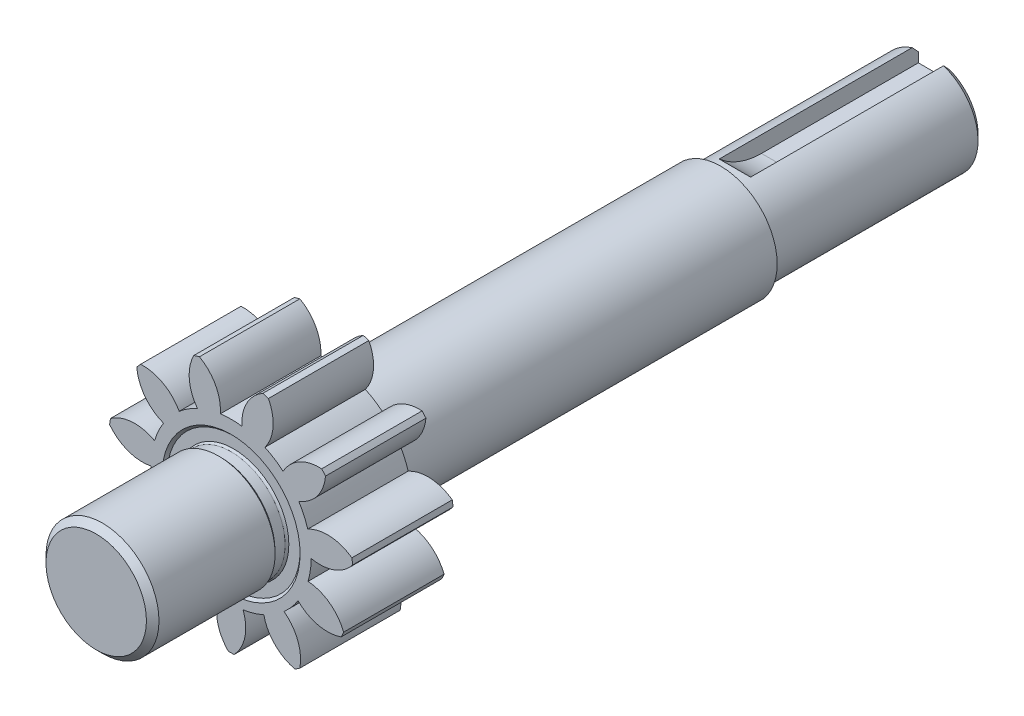
from build123d import *

# Parameters (mm, degrees)
EXTRUDE_1_DEPTH     = 16
SKETCH_2_R          = 9
EXTRUDE_2_DEPTH     = 21.5
EXTRUDE_START       = 62
SKETCH_3_R          = 9
EXTRUDE_3_DEPTH     = 62
SKETCH_4_R          = 8
EXTRUDE_4_DEPTH     = 34
CUT_EXTRUDE_1_DEPTH = 2.5
CHAMFER_1_SIZE      = 1


with BuildPart() as part:
    # 草图1 → 凸台-拉伸1 (new body)
    with BuildSketch(Plane.XY):
        with BuildLine():
            ThreePointArc((-17.539719795, -8.188913461), (-13.882626521, -8.407262966), (-10.672515451, -6.641705083))
            ThreePointArc((-10.672515451, -6.641705083), (-9.635051323, -8.016686689), (-8.421711588, -9.239271212))
            ThreePointArc((-8.421711588, -9.239271212), (-10.626145075, -12.165442895), (-10.930476691, -15.816386607))
            ThreePointArc((-10.930476691, -15.816386607), (-10.54249594, -16.072311082), (-10.148525822, -16.318915917))
            ThreePointArc((-10.148525822, -16.318915917), (-6.95393453, -14.525429313), (-5.207949909, -11.304630433))
            ThreePointArc((-5.207949909, -11.304630433), (-3.591808367, -11.900443112), (-1.910102932, -12.272965675))
            ThreePointArc((-1.910102932, -12.272965675), (-2.18258254, -15.926424664), (-0.464753394, -19.162328053))
            ThreePointArc((-0.464753394, -19.162328053), (0, -19.167867192), (0.464753394, -19.162328053))
            ThreePointArc((0.464753394, -19.162328053), (2.18258254, -15.926424664), (1.910102932, -12.272965675))
            ThreePointArc((1.910102932, -12.272965675), (3.591808367, -11.900443112), (5.207949909, -11.304630433))
            ThreePointArc((5.207949909, -11.304630433), (6.95393453, -14.525429313), (10.148525822, -16.318915917))
            ThreePointArc((10.148525822, -16.318915917), (10.54249594, -16.072311082), (10.930476691, -15.816386607))
            ThreePointArc((10.930476691, -15.816386607), (10.626145075, -12.165442895), (8.421711588, -9.239271212))
            ThreePointArc((8.421711588, -9.239271212), (9.635051323, -8.016686689), (10.672515451, -6.641705083))
            ThreePointArc((10.672515451, -6.641705083), (13.882626521, -8.407262966), (17.539719795, -8.188913461))
            ThreePointArc((17.539719795, -8.188913461), (17.737823909, -7.768459945), (17.925850869, -7.343404347))
            ThreePointArc((17.925850869, -7.343404347), (15.69598163, -4.436569144), (12.25948632, -3.166723601))
            ThreePointArc((12.25948632, -3.166723601), (12.619233563, -1.482239065), (12.748632746, 0.235364522))
            ThreePointArc((12.748632746, 0.235364522), (16.403682682, 0.485599789), (19.362176663, 2.646460979))
            ThreePointArc((19.362176663, 2.646460979), (19.301518117, 3.107272155), (19.229894055, 3.566506728))
            ThreePointArc((19.229894055, 3.566506728), (15.782454919, 4.806333783), (12.204960767, 4.016686199))
            ThreePointArc((12.204960767, 4.016686199), (11.596898309, 5.628258809), (10.777149222, 7.143157375))
            ThreePointArc((10.777149222, 7.143157375), (13.716685494, 9.329737862), (15.037279247, 12.747052577))
            ThreePointArc((15.037279247, 12.747052577), (14.7371167, 13.10191712), (14.42858175, 13.449526936))
            ThreePointArc((14.42858175, 13.449526936), (10.858110285, 12.628709513), (8.275446406, 10.030276331))
            ThreePointArc((8.275446406, 10.030276331), (6.892629782, 11.057274099), (5.383996967, 11.888498053))
            ThreePointArc((5.383996967, 11.888498053), (6.674737579, 15.317199905), (5.938151919, 18.905994868))
            ThreePointArc((5.938151919, 18.905994868), (5.493784858, 19.042245794), (5.046296687, 19.167867192))
            ThreePointArc((5.046296687, 19.167867192), (2.486392356, 16.547009024), (1.718536283, 12.964774418))
            ThreePointArc((1.718536283, 12.964774418), (0, 13.081132808), (-1.718536283, 12.964774418))
            ThreePointArc((-1.718536283, 12.964774418), (-2.486392356, 16.547009024), (-5.046296687, 19.167867192))
            ThreePointArc((-5.046296687, 19.167867192), (-5.493784858, 19.042245794), (-5.938151919, 18.905994868))
            ThreePointArc((-5.938151919, 18.905994868), (-6.674737579, 15.317199905), (-5.383996967, 11.888498053))
            ThreePointArc((-5.383996967, 11.888498053), (-6.892629782, 11.057274099), (-8.275446406, 10.030276331))
            ThreePointArc((-8.275446406, 10.030276331), (-10.858110285, 12.628709513), (-14.42858175, 13.449526936))
            ThreePointArc((-14.42858175, 13.449526936), (-14.7371167, 13.10191712), (-15.037279247, 12.747052577))
            ThreePointArc((-15.037279247, 12.747052577), (-13.716685494, 9.329737862), (-10.777149222, 7.143157375))
            ThreePointArc((-10.777149222, 7.143157375), (-11.596898309, 5.628258809), (-12.204960767, 4.016686199))
            ThreePointArc((-12.204960767, 4.016686199), (-15.782454919, 4.806333783), (-19.229894055, 3.566506728))
            ThreePointArc((-19.229894055, 3.566506728), (-19.301518117, 3.107272155), (-19.362176663, 2.646460979))
            ThreePointArc((-19.362176663, 2.646460979), (-16.403682682, 0.485599789), (-12.748632746, 0.235364522))
            ThreePointArc((-12.748632746, 0.235364522), (-12.619233563, -1.482239065), (-12.25948632, -3.166723601))
            ThreePointArc((-12.25948632, -3.166723601), (-15.69598163, -4.436569144), (-17.925850869, -7.343404347))
            ThreePointArc((-17.925850869, -7.343404347), (-17.737823909, -7.768459945), (-17.539719795, -8.188913461))
        make_face()
    extrude(amount=EXTRUDE_1_DEPTH)

    # 草图2 → 凸台-拉伸2 (add)
    with BuildSketch(Plane.XY.offset(16)):
        Circle(SKETCH_2_R)
    extrude(amount=EXTRUDE_2_DEPTH)

    # 草图3 → 凸台-拉伸3 (add)
    with BuildSketch(Plane(origin=(0, 0, 0), x_dir=(-1, 0, 0), z_dir=(0, 0, -1)).offset(EXTRUDE_START)):
        with Locations(Location((0, 0, 0), (0, 0, 180))):
            Circle(SKETCH_3_R)
    extrude(amount=-EXTRUDE_3_DEPTH)

    # 草图4 → 凸台-拉伸4 (add)
    with BuildSketch(Plane(origin=(0, 0, -62), x_dir=(-1, 0, 0), z_dir=(0, 0, -1))):
        Circle(SKETCH_4_R)
    extrude(amount=EXTRUDE_4_DEPTH)

    # 草图5 → 切除-旋转1 (revolve, cut)
    with BuildSketch(Plane(origin=(0, 0, 0), x_dir=(0, 0, -1), z_dir=(1, 0, 0)), mode=Mode.PRIVATE) as cut_revolve_1_sk:
        with BuildLine():
            Line((-16, 10.9894116), (-15.6, 10.5894116))
            Line((-15.6, 10.5894116), (-15.6, 8.792688481))
            ThreePointArc((-15.6, 8.792688481), (-15.785456972, 8.662432859), (-16, 8.5894116))
            Line((-16, 8.5894116), (-17.6, 8.5894116))
            Line((-17.6, 8.5894116), (-18, 8.9894116))
            Line((-18, 8.9894116), (-18, 10.9894116))
            Line((-18, 10.9894116), (-16, 10.9894116))
        make_face()
    cut_revolve_1 = revolve(cut_revolve_1_sk.sketch.rotate(Axis((0, 0, 37.5), (0, 0, -1)), 90), axis=Axis((0, 0, 37.5), (0, 0, -1)), mode=Mode.SUBTRACT)

    # 镜向1: 切除-旋转1 across plane
    add(cut_revolve_1.mirror(Plane.XY.offset(8)), mode=Mode.SUBTRACT)

    # 草图6 → 切除-拉伸1 (cut, symmetric)
    with BuildSketch(Plane(origin=(0, 0, 0), x_dir=(0, 0, -1), z_dir=(1, 0, 0))):
        with BuildLine():
            Line((96, 12.940111189), (96, 5))
            Line((96, 5), (71, 5))
            ThreePointArc((71, 5), (64.570358548, 7.341037224), (61.151123092, 13.268057839))
            Line((61.151123092, 13.268057839), (61.151123092, 20.241558611))
            Line((61.151123092, 20.241558611), (96, 20.241558611))
            Line((96, 20.241558611), (96, 12.940111189))
        make_face()
    extrude(amount=CUT_EXTRUDE_1_DEPTH, both=True, mode=Mode.SUBTRACT)

    # 倒角1
    chamfer_1_edges = [part.edges().sort_by_distance(p)[0] for p in [
        (-9, 0, 37.5),
        (4.69041576, -6.480740698, -96),
    ]]
    chamfer(chamfer_1_edges, length=CHAMFER_1_SIZE)


solid = part.part
